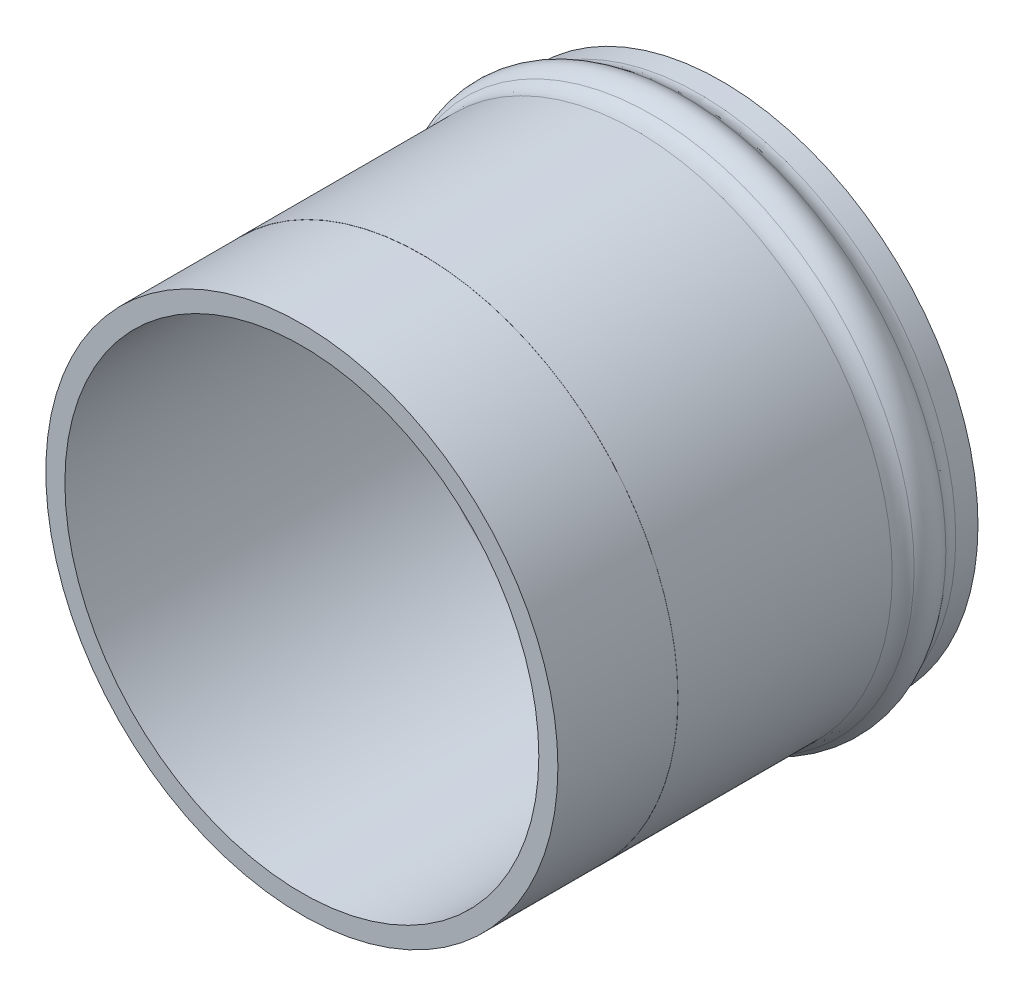
SolidWorks part; units mm, degrees
material "STKM11A"
ref_plane "Front Plane" through (0, 0, 0) normal (0, 0, 1) x (1, 0, 0)
ref_plane "Top Plane" through (0, 0, 0) normal (0, 1, 0) x (1, 0, 0)
ref_plane "Right Plane" through (0, 0, 0) normal (1, 0, 0) x (0, 0, -1)
sketch "Sketch1" plane through (0, 0, 0) normal (1, 0, 0) x (0, 0, -1)
  line L0 (0, 0) -> (35, 0) construction
  line L1 (0, 21.35) -> (27.8542, 21.35)
  line L2 (33.1458, 21.35) -> (35, 21.35)
  arc A0 (31.8229, 21.85) -> (29.1771, 21.85) centre (30.5, 20.35) ccw
  arc A1 (33.1458, 21.35) -> (31.8229, 21.85) centre (33.1458, 23.35) cw
  arc A2 (27.8542, 21.35) -> (29.1771, 21.85) centre (27.8542, 23.35) ccw
  point P10 (32.2321, 21.35)
  point P13 (28.7679, 21.35)
  dimension "D1" = 4
  dimension "D2" = 2
  dimension "D7" = 1
  dimension "D3" = 35
  dimension "D4" = 42.7
  dimension "D5" = 1
  dimension "D6" = 4.5
revolve "Revolve-Thin1" add sketch "Sketch1" angle 360 about L0
sketch "Sketch2" plane through (0, 0, 0) normal (0, 0, 1) x (1, 0, 0)
  circle A0 centre (0, 0) radius 21.35
  circle A1 centre (0, 0) radius 21.34
  dimension "D1" = 42.7
  dimension "D2" = 0.01
extrude "Cut-Extrude1" cut sketch "Sketch2" against normal blind 10
